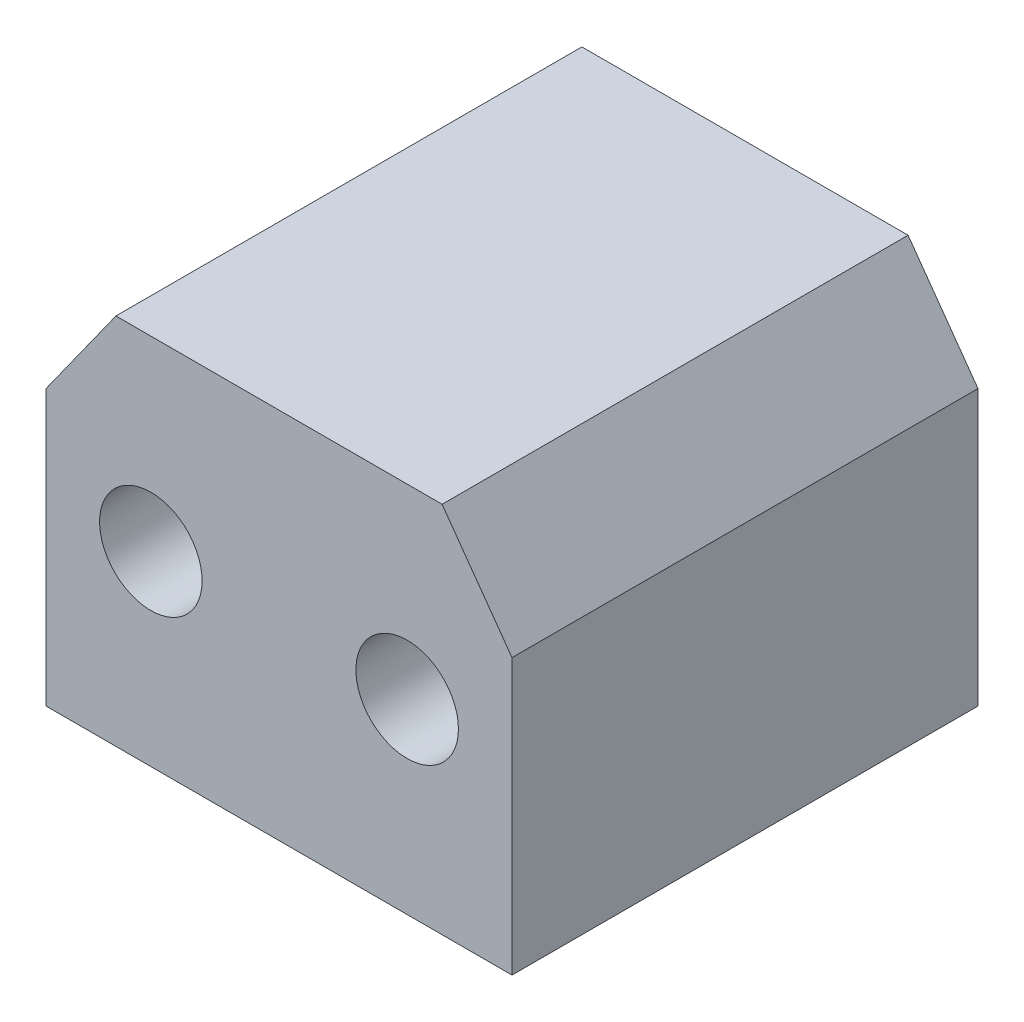
SolidWorks part; units mm, degrees
material "Q235B"
ref_plane "Front Plane" through (0, 0, 0) normal (0, 0, 1) x (1, 0, 0)
ref_plane "Top Plane" through (0, 0, 0) normal (0, 1, 0) x (1, 0, 0)
ref_plane "Right Plane" through (0, 0, 0) normal (1, 0, 0) x (0, 0, -1)
sketch "Sketch1" plane through (0, 0, 0) normal (0, 0, 1) x (1, 0, 0)
  line L1 (50, -40) -> (-50, -40)
  line L2 (50, -40) -> (50, 40)
  line L3 (50, 40) -> (-50, 40)
  line L4 (-50, -40) -> (-50, 40)
  line L5 (50, -40) -> (-50, 40) construction
  line L6 (50, 40) -> (-50, -40) construction
  point P0 (0, 0)
  dimension "D1" = 80
  dimension "D2" = 100
extrude "Boss-Extrude1" add sketch "Sketch1" along normal blind 100
chamfer "Chamfer1" distance 10 angle 45 2 edges at (-50, 40, 50) (50, 40, 50)
hole_wizard "Ø22 diameter hole1" positions "Sketch2" profile "Sketch3" hole size "Ø12.0" standard "GB" end condition up to next
sketch "Sketch2" plane through (0, 0, 100) normal (0, 0, 1) x (1, 0, 0)
  line L0 (0, 40) -> (0, -40) construction
  line L1 (40, 40) -> (-40, 40) construction
  line L2 (-50, -40) -> (50, -40) construction
  point P0 (-27.5, 0)
  point P10 (27.5, 0)
  dimension "D1" = 55
  dimension "D2" = 40
sketch "Sketch3" plane through (-27.5, 0, 100) normal (1, 0, 0) x (0, -1, 0)
  line L0 (0, 0) -> (0, 100)
  line L1 (0, 100) -> (11, 100)
  line L2 (11, 100) -> (11, 0)
  line L5 (11, 0) -> (0, 0)
  line L11 (0, -6.35) -> (0, 107.95) construction
  dimension "通孔孔直径" = 22
  dimension "通孔孔深度" = 100
sketch "Sketch4" plane through (0, 0, 100) normal (0, 0, 1) x (1, 0, 0)
  line L0 (-35, 40) -> (-50, 19)
  line L1 (40, 40) -> (-40, 40) construction
  line L2 (-50, 30) -> (-50, -40) construction
  line L3 (-50, 19) -> (-50, 40)
  line L4 (-50, 40) -> (-35, 40)
  line L5 (0, 40) -> (0, 0) construction
  line L6 (50, 40) -> (35, 40)
  line L7 (50, 19) -> (50, 40)
  line L8 (35, 40) -> (50, 19)
  line L9 (-50, -40) -> (50, -40) construction
  dimension "D1" = 70
  dimension "D2" = 59
extrude "Cut-Extrude1" cut sketch "Sketch4" against normal through all both and the other way through all
